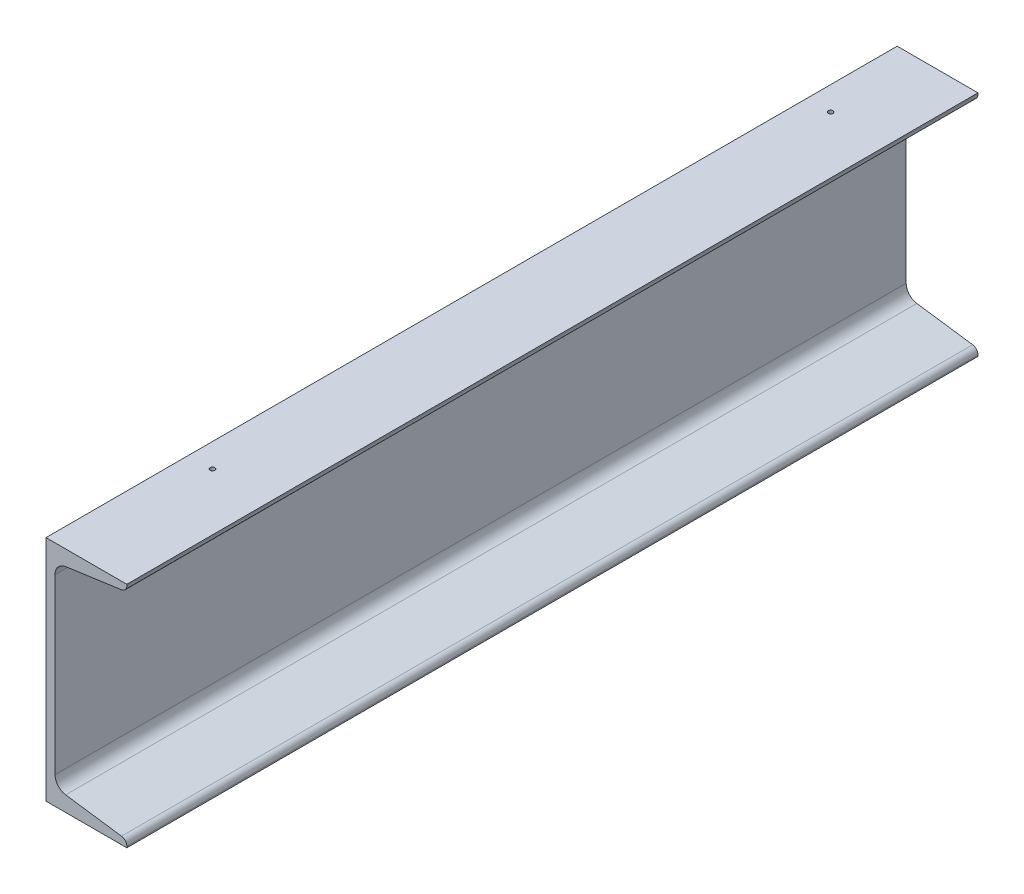
SolidWorks part; units mm, degrees
material "1023 碳钢板 (SS)"
ref_plane "前视基准面" through (0, 0, 0) normal (0, 0, 1) x (1, 0, 0)
ref_plane "上视基准面" through (0, 0, 0) normal (0, 1, 0) x (1, 0, 0)
ref_plane "右视基准面" through (0, 0, 0) normal (1, 0, 0) x (0, 0, -1)
sketch "草图1" plane through (0, 0, 0) normal (0, 0, 1) x (1, 0, 0)
  line L0 (0, 0) -> (-85, 0)
  line L1 (-85, 0) -> (-85, -240)
  line L2 (-85, -240) -> (0, -240)
  line L3 (0, -240) -> (0, -238.6233)
  line L4 (-5.5954, -232.1866) -> (-64.3093, -223.9349)
  line L5 (-75.5, -211.0614) -> (-75.5, -28.9386)
  line L6 (-64.3093, -16.0651) -> (-5.5954, -7.8134)
  line L7 (0, -1.3767) -> (0, 0)
  line L8 (-42.5, -227) -> (-42.5, -240) construction
  arc A0 (-64.3093, -223.9349) -> (-75.5, -211.0614) centre (-62.5, -211.0614) cw
  arc A1 (-75.5, -28.9386) -> (-64.3093, -16.0651) centre (-62.5, -28.9386) cw
  arc A2 (0, -238.6233) -> (-5.5954, -232.1866) centre (-6.5, -238.6233) ccw
  arc A3 (-5.5954, -7.8134) -> (0, -1.3767) centre (-6.5, -1.3767) ccw
  dimension "D7" = 13
  dimension "D8" = 6.5
  dimension "D1" = 240
  dimension "D2" = 85
  dimension "D3" = 42.5
  dimension "D4" = 13
  dimension "D5" = 9.5
  dimension "D6" = 8
extrude "凸台-拉伸1" add sketch "草图1" along normal blind 895 contours A3 L6 A1 L5 A0 L4 A2 L3 L2 L1 L0 L7
sketch "草图2" plane through (-85, 0, 0) normal (-1, 0, 0) x (0, 0, 1)
  line L0 (895, 0) -> (0, 0) construction
  line L2 (0, -211.0614) -> (0, -28.9386) construction
  circle A0 centre (2840, -126) radius 10
  circle A1 centre (2840, -196) radius 10
  circle A2 centre (2640, -126) radius 10
  circle A3 centre (2640, -196) radius 10
  circle A4 centre (2440, -126) radius 10
  circle A5 centre (2440, -196) radius 10
  circle A6 centre (2240, -126) radius 10
  circle A7 centre (2240, -196) radius 10
  circle A8 centre (2040, -126) radius 10
  circle A9 centre (2040, -196) radius 10
  circle A10 centre (1840, -126) radius 10
  circle A11 centre (1840, -196) radius 10
  circle A12 centre (1640, -126) radius 10
  circle A13 centre (1640, -196) radius 10
  circle A14 centre (1440, -126) radius 10
  circle A15 centre (1440, -196) radius 10
  circle A16 centre (1240, -126) radius 10
  circle A17 centre (1240, -196) radius 10
  circle A18 centre (1040, -126) radius 10
  circle A19 centre (1040, -196) radius 10
  circle A20 centre (840, -126) radius 10
  circle A21 centre (840, -196) radius 10
  circle A22 centre (640, -126) radius 10
  circle A23 centre (640, -196) radius 10
  circle A24 centre (440, -126) radius 10
  circle A25 centre (440, -196) radius 10
  circle A26 centre (240, -126) radius 10
  circle A27 centre (240, -196) radius 10
  dimension "D3" = 240
  dimension "D4" = 20
  dimension "D1" = 70
  dimension "D2" = 126
  dimension "D5" = 14
sketch "草图9" plane through (0, 0, 0) normal (0, 1, 0) x (1, 0, 0)
  line L1 (-85, -895) -> (-85, 0) construction
  line L2 (0, -895) -> (-85, -895) construction
  circle A0 centre (-60, -95) radius 6
  circle A1 centre (-60, -745) radius 6
  point P8 (0, 0)
  dimension "D2" = 650
  dimension "D3" = 25
  dimension "D4" = 12
  dimension "D1" = 150
hole_wizard "M6 螺纹孔1" positions "草图10" profile "草图11" tap size "M6" standard "ISO"
sketch "草图10" plane through (0, 0, 0) normal (0, 1, 0) x (1, 0, 0)
  point P0 (-60, -745)
  point P3 (-60, -95)
sketch "草图11" plane through (-60, 0, 745) normal (1, 0, 0) x (0, 0, 1)
  line L0 (0, 0) -> (0, 16.5022)
  line L1 (0, 16.5022) -> (2.5, 15)
  line L2 (2.5, 15) -> (2.5, 0)
  line L5 (2.5, 0) -> (0, 0)
  line L10 (0, 16.5022) -> (-2.5, 15) construction
  line L11 (0, -6.35) -> (0, 107.95) construction
  dimension "螺纹孔钻头直径" = 5
  dimension "螺纹孔钻头深度" = 15
  dimension "导头角度" = 118
cosmetic thread "孔螺蚊线3"
cosmetic thread "孔螺蚊线4"
